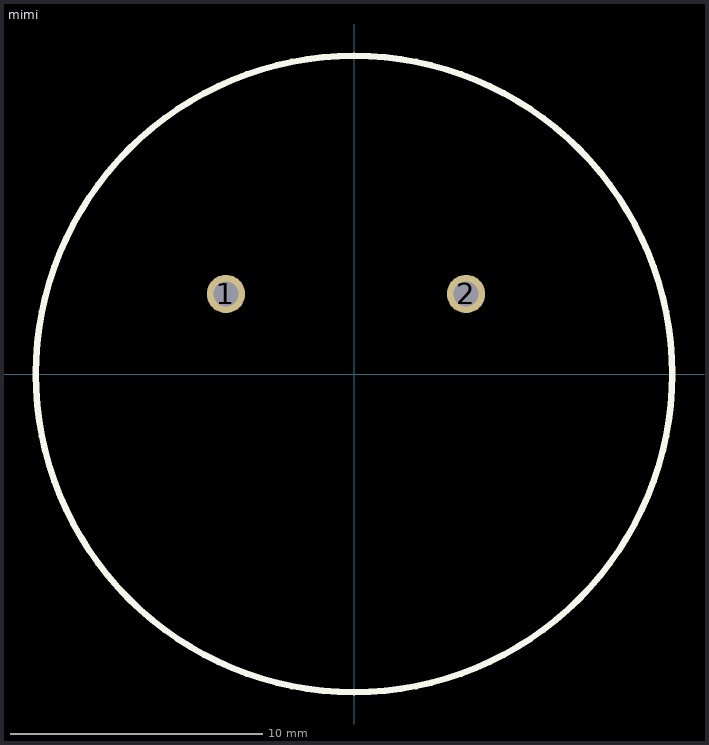
[diagram p0: the footprint, top view; thin cyan lines are the x and y axes]
# Altium footprint library MISC86340-21.PcbLib: 1 footprints
Each footprint in its own frame and in the unit in brackets; x right, y up, seen from the top. Pads: shape width x height; smd on the part's side, far side on the other; paste and mask are expansions set on the pad; w line width, h text height; cw(c..) or ccw(c..) is an arc to the next point about the centre after c.

## mimi [mil]
pads (2):
  round 60 hole 39.37: 1(-200,125) 2(175,125)
Top Overlay:
  circle w10: c0,0 r497.02